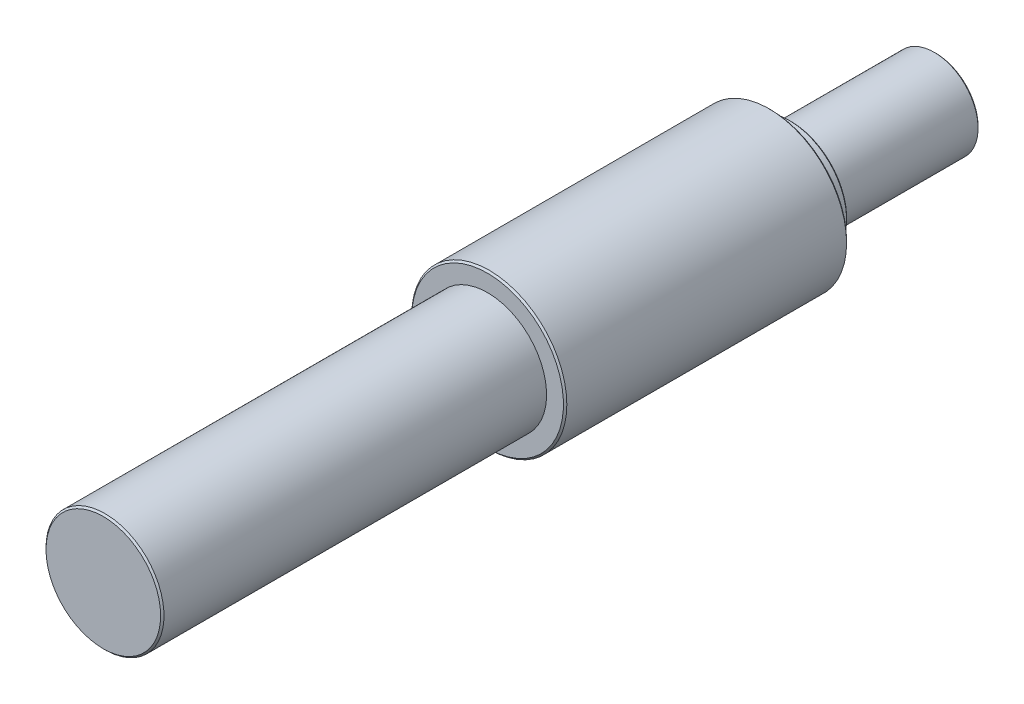
SolidWorks part; units mm, degrees
material "AL6061"
ref_plane "前视基准面" through (0, 0, 0) normal (0, 0, 1) x (1, 0, 0)
ref_plane "上视基准面" through (0, 0, 0) normal (0, 1, 0) x (1, 0, 0)
ref_plane "右视基准面" through (0, 0, 0) normal (1, 0, 0) x (0, 0, -1)
sketch "草图1" plane through (0, 0, 0) normal (0, 0, 1) x (1, 0, 0)
  circle A0 centre (0, 0) radius 17.5
extrude "凸台-拉伸1" add sketch "草图1" along normal mid plane 114
sketch "草图2" plane through (0, 0, -57) normal (0, 0, -1) x (-1, 0, 0)
  circle A0 centre (0, 0) radius 23
extrude "凸台-拉伸2" add sketch "草图2" along normal blind 84
sketch "草图3" plane through (0, 0, -141) normal (0, 0, -1) x (-1, 0, 0)
  circle A0 centre (0, 0) radius 17
extrude "凸台-拉伸3" add sketch "草图3" along normal blind 6
sketch "草图4" plane through (0, 0, -147) normal (0, 0, -1) x (-1, 0, 0)
  circle A0 centre (0, 0) radius 13
extrude "凸台-拉伸4" add sketch "草图4" along normal blind 43
chamfer "倒角1" distance 0.5 angle 45 5 edges at (-13, 0, -190) (-23, 0, -141) (-17, 0, -147) (-23, 0, -57) (17.5, 0, 57)
